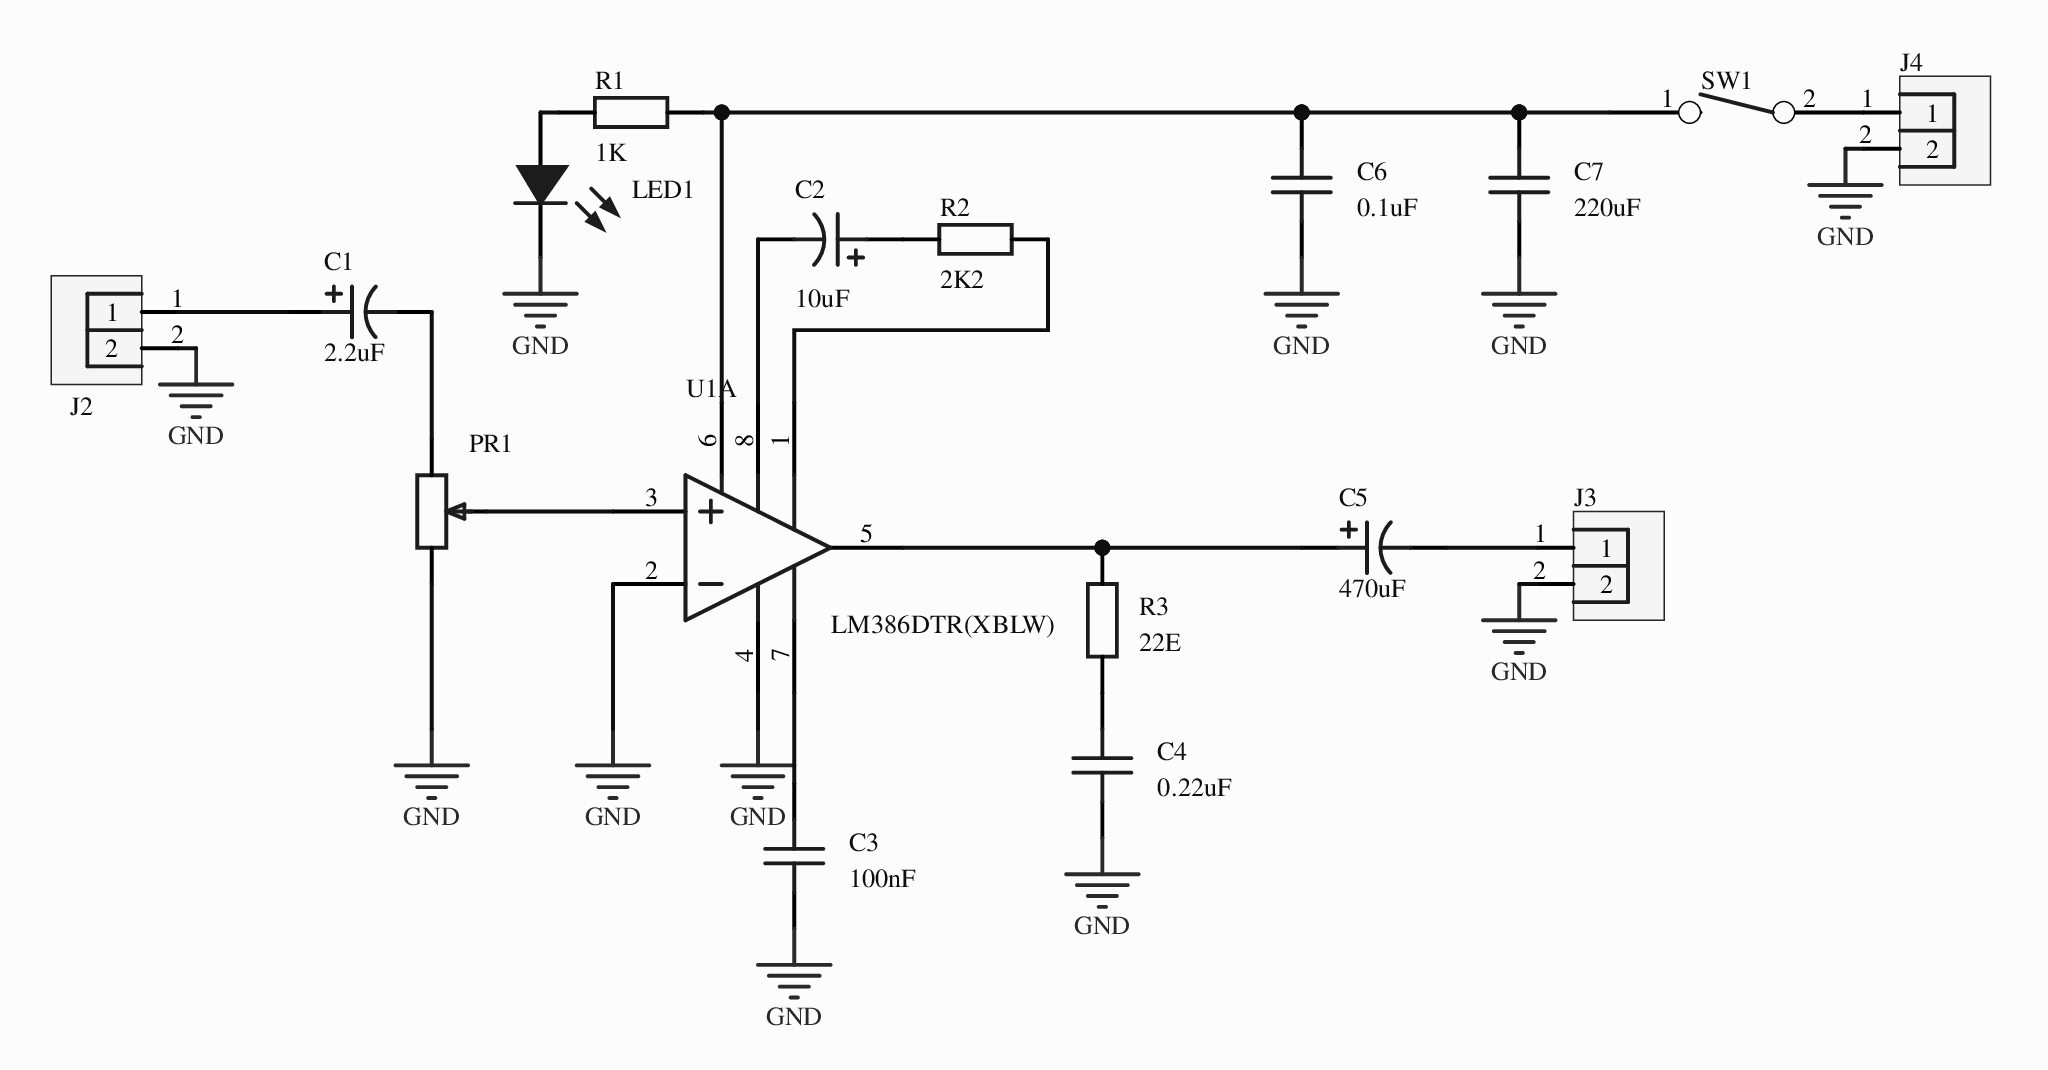
[diagram p0: MISC52147-3.schdoc]
# Altium project MISC52147-2.PrjPcb
1 sheet, 17 parts. Net scope: global (net labels, ports and power ports of the same name join across sheets).
Board file: MISC52147.pcbdoc

## Sheet MISC52147-3.schdoc
size 210 x 148 mm; Version: V1.0; @Project Name: MISC52147; @Update Date: 2026-10-07; @Create Date: 2026-10-07; @Board Name: MISC52147; @Create Time: 12:44:54; @Page Count: 1; @Page No: 1; @Schematic Name: MISC52147; @Update Time: 12:44:54; Size: A4

### Parts
C1  2.2uF  [CAP-TH_BD5.0-P2.00-D0.8-FD-10UF50VC110GL]
C2  10uF  [CAP-TH_BD5.0-P2.00-D0.8-FD-10UF50VC110GL]
C3  100nF  [C0603]
C4  0.22uF  [C0603]
C5  470uF  [CAP-TH_BD5.0-P2.00-D0.8-FD-10UF50VC110GL]
C6  0.1uF  [C0603]
C7  220uF  [C0603]
J2  (no value)  [HDR-TH_2P-P2.54-V-M-1]
J3  (no value)  [HDR-TH_2P-P2.54-V-M-1]
J4  (no value)  [HDR-TH_2P-P2.54-V-M-1]
LED1  (no value)  [LED_0603]
PR1  10kΩ  [R_3296]  (value not drawn)
R1  1K  [R0603]
R2  2K2  [R0603]
R3  22E  [R0603]
SW1  (no value)  [拨动开关_侧]
U1  LM386DTR(XBLW)  [SOP-8_L4.9-W3.9-P1.27-LS6.0-BL]  (part A of 2)

### Nets
GND: C3.1 C4.1 C6.1 C7.1 J2.2 J3.2 J4.2 LED1.1(C) PR1.1 U1.2(IN-) U1.4(GND)
NetC1_1: C1.1 J2.1
NetC1_2: C1.2 PR1.3
NetC2_1: C2.1 R2.1
NetC2_2: C2.2 U1.8(VCC)
NetC3_2: C3.2 U1.7(GND)
NetC4_2: C4.2 R3.1
NetC5_1: C5.1 R3.2 U1.5(VOUT)
NetC5_2: C5.2 J3.1
NetC6_2: C6.2 C7.2 R1.2 SW1.1 U1.6(GND)
NetJ4_1: J4.1 SW1.2
NetLED1_2: LED1.2(A) R1.1
NetPR1_2: PR1.2 U1.3(IN+)
NetR2_2: R2.2 U1.1(GND)

### Library data of the parts
C1 C2 C5 = 10UF50VC110GL: 容值:10uF;精度:±20%;额定电压:50V;纹波电流:120mA@100KHz;等效串联电阻(ESR):1.6Ω;; Manufacturer: Econd(米朗电子); 3D Model: b35ab6b0460c4c43a629d91cfc2b58780819f05c4eef4c71ace90d822a990e87; 3D Model Transform: 196.85,196.85,0,0,0,0,0,0,-196.85; Tolerance: ±20%; Voltage Rating: 50V; Equivalent Series Resistance(ESR): 1.6Ω; Pin Spacing: 2mm; Lifetime: 5000hrs@105℃; AddInBom: yes; Symbol: 10UF50VC110GL; Device: 10UF50VC110GL; LCSC Part Name: 10uF ±20% 50V; Manufacturer Part: 10UF50VC110GL; Supplier Footprint: 插件,D5xL11mm; JLCPCB Part Class: Extended Part; Datasheet: https://item.szlcsc.com/datasheet/10UF50VC110GL/49031974.html; Supplier: LCSC; Ripple Current: 120mA@100KHz; Diameter: 5mm; Height - Seated (Max): 11mm; Operating Temperature: -40℃~+105℃; FootprintName: CAP-TH_BD5.0-P2.00-D0.8-FD-10UF50VC110GL; ConvertToPcb: yes; ModelName: CAP-TH_BD5.0-P2.00-D0.8-FD-10UF50VC110GL
  C1: Value: 2.2uF
  C2: Supplier Part: C46867109; Value: 10uF
  C5: Value: 470uF
C3 C4 C6 C7 = CAP_0603: Symbol: Capacitance; ConvertToPcb: yes; ModelId: ac125912035d415993ca9572d50418b10819f05c4eef4c71ace90d822a990e87; ModelName: C0603_L1.6-W0.8-H0.8; ModelTransform: 62.992,31.496,0,0,0,0,0,0,0; Device: CAP_0603; FootprintName: C0603; AddInBom: yes; Supplier Footprint: 0603
  C3: Value: 100nF
  C4: Value: 0.22uF
  C6: Value: 0.1uF
  C7: Value: 220uF
J2-J4 = HDR-M_2.54_1x2P: Symbol: 210S-1*2P L=11.6MMGold-plated black; 3D Model: 79b2e9f2d70a4d68a1b7098f27c6d4c50819f05c4eef4c71ace90d822a990e87; 3D Model Transform: 200,100,0,0,0,0,0,0,-118.11; ConvertToPcb: yes; ModelName: HDR-M-2.54_1x2; Device: HDR-M_2.54_1x2P; Supplier Part: C124375; Supplier Footprint: 插件; FootprintName: HDR-TH_2P-P2.54-V-M-1; AddInBom: yes
LED1 = LED_0603-B: Symbol: LED_B; Convert to PCB: yes; 3D Model: eb8d964598f24248affda46f619856c50819f05c4eef4c71ace90d822a990e87; 3D Model Transform: 63.1,31.6,23.7,0,0,0,0,0,0; ModelName: LED-0603_B; Device: LED_0603-B; Add into BOM: yes; Supplier Footprint: 0603; FootprintName: LED_0603
PR1 = R_3296: ConvertToPcb: yes; ModelId: b182808559bb43bda9e7de64b64134cb0819f05c4eef4c71ace90d822a990e87; ModelName: 3296W; ModelTransform: 373.98,188.96,590.49,180,0,0,0,0,-140; Symbol: R_3296; Device: R_3296; FootprintName: R_3296; AddInBom: yes; Supplier Footprint: 直插; Value: 10kΩ
R1-R3 = Res_0603: Symbol: 电阻; 3D Model: fc143cca1e79419f9cd78b61e9279f080819f05c4eef4c71ace90d822a990e87; 3D Model Transform: 31.8897,63.7794,0,90,0,0,0,0,0; ConvertToPcb: yes; Device: Res_0603; Supplier Footprint: 0603; FootprintName: R0603; AddInBom: yes; ModelName: R0603
  R1: Value: 1K
  R2: Value: 2K2
  R3: Value: 22E
SW1 = 拨动开关_侧: Symbol: 拨动开关; ConvertToPcb: yes; ModelId: 10ea2cc5ba004a75b38812aadef1031f0819f05c4eef4c71ace90d822a990e87; ModelName: SW-TH_SK-12D07-VG3; ModelTransform: 337.98,287.46,295.24,0,0,0,0,-57,-110; Device: 拨动开关_侧; FootprintName: 拨动开关_侧; AddInBom: yes; Supplier Footprint: 插件
U1 = LM386DTR(XBLW): 功放类型:-;扬声器通道数:-;输出功率:-;静态电流(Iq):4mA;; Manufacturer: XBLW(芯伯乐); Relevance: []; AddInBom: yes; ModelId: 75c24a7891ee4dd6bdac16a7163ff87e0819f05c4eef4c71ace90d822a990e87; ModelName: SOP-8_L4.9-W3.9-P1.27-LS6.0-BL-1; ModelTransform: 192.913,236.22,0,0,0,0,-0.393,2.749,0; Total Harmonic Distortion + Noise (THD+N): 0.2%; Quiescent Current: 4mA; Power Supply Rejection Ratio (PSRR): 50dB; Voltage - Supply: 4V~12V; Symbol: LM386DTR(XBLW); Device: LM386DTR(XBLW); FootprintName: SOP-8_L4.9-W3.9-P1.27-LS6.0-BL; LCSC Part Name: 低电压音频功率放大器，多用于低压消费类音频产品; SupplierPart: C42395500; ManufacturerPart: LM386DTR(XBLW); Supplier Footprint: SOP-8; JLCPCB Part Class: Extended Part; Datasheet: https://item.szlcsc.com/datasheet/LM386DTR(XBLW)/44341334.html; Supplier: LCSC; ConvertToPcb: yes; Class: -; Speaker Channels: -; Output Power: -; Signal-to-Noise Ratio: -; Efficiency: -; Number of Inputs: -; Features: 模拟电压增益; Operating Temperature: 0℃~+70℃